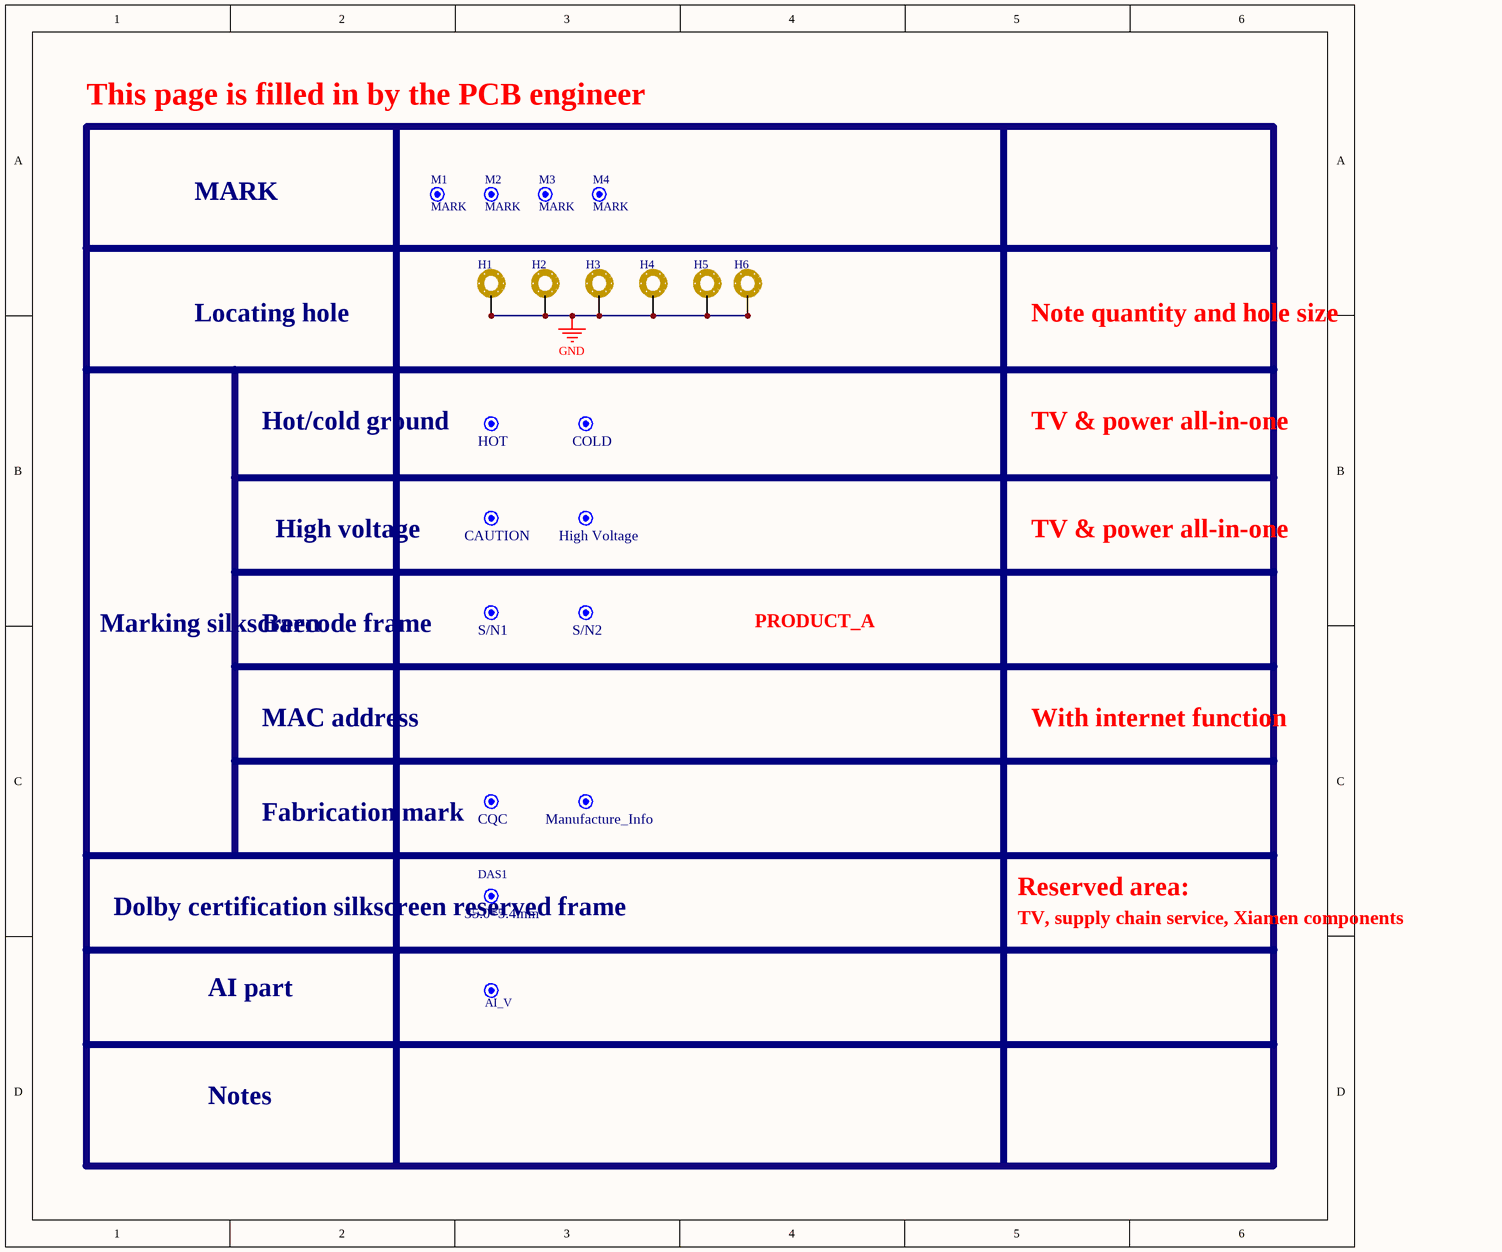
[diagram p0: MISC86383-4.SchDoc]
# Altium schematic sheet MISC86383-4.SchDoc
size 254 x 233 mm

## Parts
AI_V  AI_GRIPPER_V  [AI_GRIPPER_V]  (value not drawn)
CAUTION  CAUTION  [CAUTION]
COLD  COLD  [COLD]
CQC  CQC  [CQC]
DAS1  35.0*5.4mm  [DOLBY_AS2]
H1  Location hole  [ASSE4.0C-3]  (value not drawn)
H2  Location hole  [ASSE4.0C-3]  (value not drawn)
H3  Location hole  [ASSE4.0C-3]  (value not drawn)
H4  Location hole  [ASSE4.0C-3]  (value not drawn)
H5  Location hole  [ASSE4.0C-3]  (value not drawn)
H6  Location hole  [ASSE4.0C-3]  (value not drawn)
High_Voltage  High Voltage  [High Voltage]
HOT  HOT  [HOT]
M1  MARK  [MARK]
M2  MARK  [MARK]
M3  MARK  [MARK]
M4  MARK  [MARK]
Manufacture_Info  Manufacture_Info  [Manufacture_Info]
S/N1  Barcode  [Barcode]  (value not drawn)
S/N2  Barcode  [Barcode]  (value not drawn)

## Nets
GND: H1.1 H1.2 H1.3 H1.4 H1.5 H1.6 H2.1 H2.2 H2.3 H2.4 H2.5 H2.6 H3.1 H3.2 H3.3 H3.4 H3.5 H3.6 H4.1 H4.2 H4.3 H4.4 H4.5 H4.6 H5.1 H5.2 H5.3 H5.4 H5.5 H5.6 H6.1 H6.2 H6.3 H6.4 H6.5 H6.6

## Notes on the sheet
- This page is filled in by the PCB engineer
- MARK
- Locating hole
- Note quantity and hole size
- (near HOT) Hot/cold ground
- TV & power all-in-one
- High voltage
- Marking silkscreen
- Barcode frame
- PRODUCT_A
- MAC address
- With internet function
- (near CQC) Fabrication mark
- (near DAS1) Dolby certification silkscreen reserved frame
- Reserved area:
- TV, supply chain service, Xiamen components
- AI part
- Notes

## Library data of the parts
DAS1 = DOLBY_AS2
H1-H6 = Location hole-D
M1-M4 = MARK-D